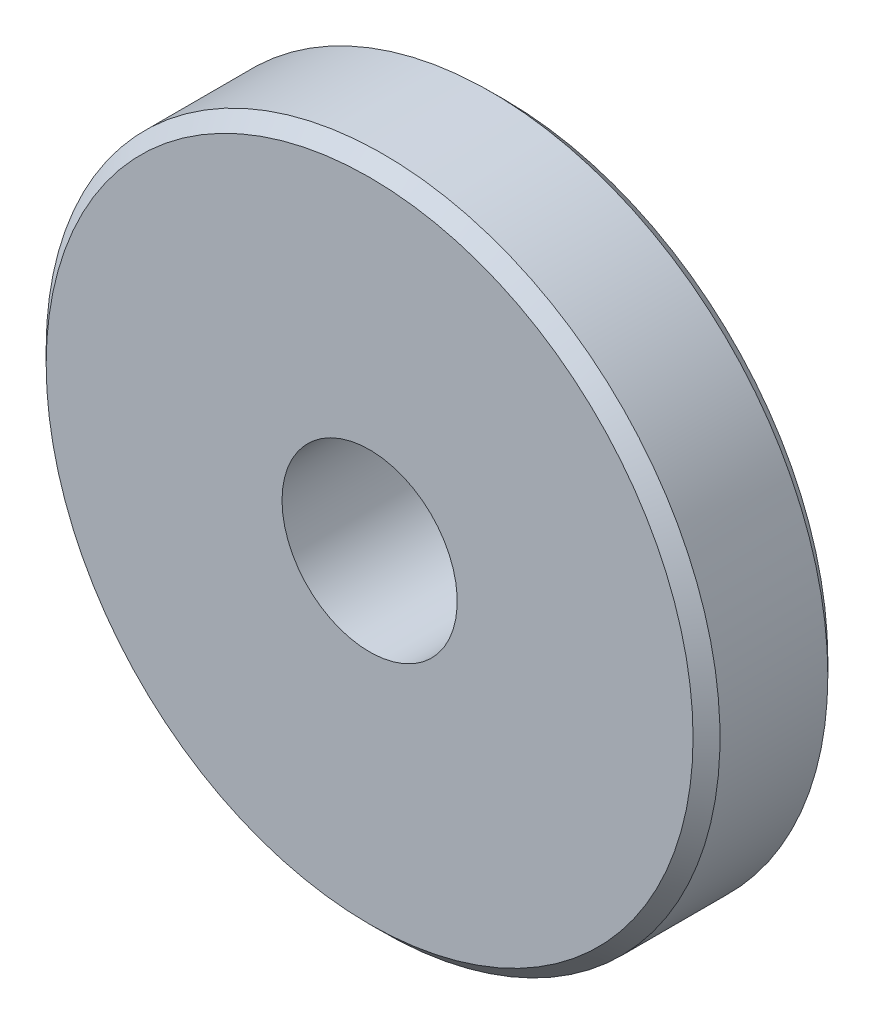
from build123d import *

# Parameters (mm, degrees)
SKETCH_1_R      = 12.5
SKETCH_1_R_2    = 3.25
EXTRUDE_1_DEPTH = 2.5
CHAMFER_1_SIZE  = 0.5


with BuildPart() as part:
    # 草图1 → 凸台-拉伸1 (new, symmetric)
    with BuildSketch(Plane.XY):
        Circle(SKETCH_1_R)
        Circle(SKETCH_1_R_2, mode=Mode.SUBTRACT)
    extrude(amount=EXTRUDE_1_DEPTH, both=True)

    # 倒角1
    chamfer_1_edges = [part.edges().sort_by_distance(p)[0] for p in [
        (-12.5, 0, -2.5),
        (-12.5, 0, 2.5),
    ]]
    chamfer(chamfer_1_edges, length=CHAMFER_1_SIZE)


solid = part.part
